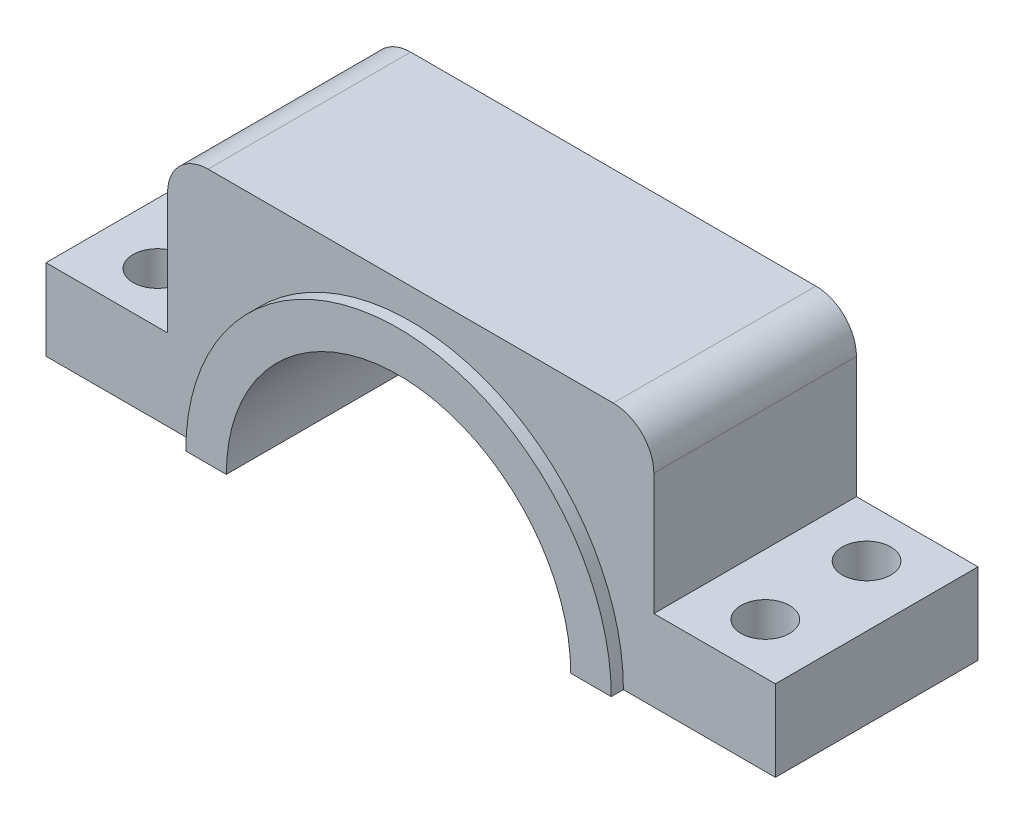
from build123d import *

# Parameters (mm, degrees)
SKETCH_1_W          = 120
SKETCH_1_H          = 50
EXTRUDE_1_DEPTH     = 60
SKETCH_2_R          = 42.5
CUT_EXTRUDE_1_DEPTH = 60
SKETCH_3_W          = 30
SKETCH_3_H          = 50
EXTRUDE_2_DEPTH     = 20
FILLET_1_R          = 10
EXTRUDE_START       = 3
EXTRUDE_3_DEPTH     = 3
SKETCH_5_R          = 6
CUT_EXTRUDE_2_DEPTH = 67


with BuildPart() as part:
    # 草图1 → 凸台-拉伸1 (new body)
    with BuildSketch(Plane(origin=(0, 0, 0), x_dir=(1, 0, 0), z_dir=(0, 1, 0))):
        Rectangle(SKETCH_1_W, SKETCH_1_H)
    extrude(amount=EXTRUDE_1_DEPTH)

    # 草图2 → 切除-拉伸1 (cut)
    with BuildSketch(Plane.XY.offset(25)):
        Circle(SKETCH_2_R)
    extrude(amount=-CUT_EXTRUDE_1_DEPTH, mode=Mode.SUBTRACT)

    # 草图3 → 凸台-拉伸2 (add)
    with BuildSketch(Plane.XZ):
        with Locations((-75, 0)):
            Rectangle(SKETCH_3_W, SKETCH_3_H)
        with Locations((75, 0)):
            Rectangle(SKETCH_3_W, SKETCH_3_H)
    extrude(amount=-EXTRUDE_2_DEPTH)

    # 圆角1
    fillet_1_edges = [part.edges().sort_by_distance(p)[0] for p in [
        (-60, 60, 0),
        (60, 60, 0),
    ]]
    fillet(fillet_1_edges, radius=FILLET_1_R)

    # 草图4 → 凸台-拉伸3 (add)
    with BuildSketch(Plane.XY.offset(25).offset(EXTRUDE_START)):
        with BuildLine():
            Line((-52.5, 0), (-42.5, 0))
            ThreePointArc((-42.5, 0), (0, 42.5), (42.5, 0))
            Line((42.5, 0), (52.5, 0))
            ThreePointArc((52.5, 0), (0, 52.5), (-52.5, 0))
        make_face()
    extrude_3 = extrude(amount=-EXTRUDE_3_DEPTH)

    # 镜向1: 凸台-拉伸3 across plane
    add(extrude_3.mirror(Plane.XY))

    # 草图5 → 切除-拉伸2 (cut)
    with BuildSketch(Plane(origin=(0, 20, 0), x_dir=(1, 0, 0), z_dir=(0, 1, 0))):
        with Locations(Location((75, 12.5, 0), (0, 0, 270))):
            Circle(SKETCH_5_R)
        with Locations(Location((75, -12.5, 0), (0, 0, 270))):
            Circle(SKETCH_5_R)
        with Locations(Location((-75, -12.5, 0), (0, 0, 270))):
            Circle(SKETCH_5_R)
        with Locations(Location((-75, 12.5, 0), (0, 0, 270))):
            Circle(SKETCH_5_R)
    extrude(amount=-CUT_EXTRUDE_2_DEPTH, mode=Mode.SUBTRACT)


solid = part.part
